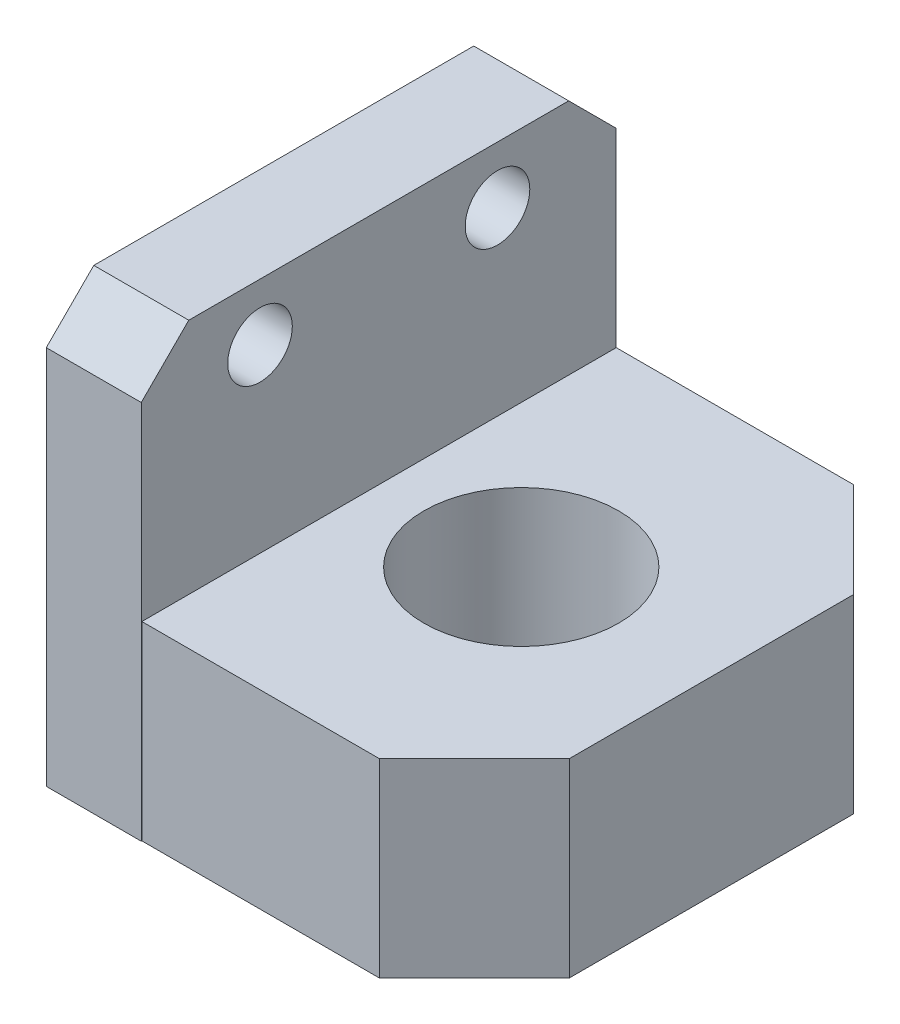
SolidWorks part; units mm, degrees
ref_plane "前视基准面" through (0, 0, 0) normal (0, 0, 1) x (1, 0, 0)
ref_plane "上视基准面" through (0, 0, 0) normal (0, 1, 0) x (1, 0, 0)
ref_plane "右视基准面" through (0, 0, 0) normal (1, 0, 0) x (0, 0, -1)
sketch "草图1" plane through (0, 0, 0) normal (1, 0, 0) x (0, 0, -1)
  line L1 (-25, 22.5) -> (25, 22.5)
  line L2 (-25, 22.5) -> (-25, -22.5)
  line L3 (-25, -22.5) -> (25, -22.5)
  line L4 (25, 22.5) -> (25, -22.5)
  line L5 (-25, 22.5) -> (25, -22.5) construction
  line L6 (-25, -22.5) -> (25, 22.5) construction
  point P0 (0, 0)
  dimension "D1" = 50
  dimension "D2" = 45
extrude "凸台-拉伸1" add sketch "草图1" along normal blind 10
sketch "草图2" plane through (10, 0, 0) normal (1, 0, 0) x (0, 0, -1)
  line L0 (25, -22.5) -> (25, 22.5) construction
  line L1 (-24.9382, -2.5) -> (25, -2.5)
  line L2 (-24.9382, -2.5) -> (-24.9382, -22.5)
  line L3 (-24.9382, -22.5) -> (25, -22.5)
  line L4 (25, -2.5) -> (25, -22.5)
  line L5 (-24.9382, -2.5) -> (25, -22.5) construction
  line L6 (-24.9382, -22.5) -> (25, -2.5) construction
  line L7 (-25, -22.5) -> (25, -22.5) construction
  dimension "D2" = 20
extrude "凸台-拉伸2" add sketch "草图2" along normal blind 35
hole_wizard "Ø20.5 (20.5) 直径孔1" positions "草图3" profile "草图4" hole size "Ø20.5" standard "GB" end condition through all
sketch "草图3" plane through (0, -22.5, 0) normal (0, -1, 0) x (-1, 0, 0)
  point P0 (-25, 0)
  dimension "D1" = 25
sketch "草图4" plane through (25, -22.5, 0) normal (1, 0, 0) x (0, 0, -1)
  line L0 (0, 0) -> (0, 45)
  line L1 (0, 45) -> (10.25, 45)
  line L2 (10.25, 45) -> (10.25, 0)
  line L5 (10.25, 0) -> (0, 0)
  line L11 (0, -6.35) -> (0, 107.95) construction
  dimension "通孔孔直径" = 20.5
  dimension "通孔孔深度" = 45
hole_wizard "M8 螺纹孔1" positions "草图5" profile "草图6" tap size "M8" standard "GB"
sketch "草图5" plane through (10, 0, 0) normal (1, 0, 0) x (0, 0, -1)
  line L0 (0, 27.2455) -> (0, 0) construction
  line L2 (25, 22.5) -> (-25, 22.5) construction
  point P0 (-12.5, 16.5)
  point P2 (12.5, 16.5)
  point P4 (-12.5, -13.5)
  point P6 (12.5, -13.5)
  dimension "D1" = 25
  dimension "D2" = 30
  dimension "D3" = 6
sketch "草图6" plane through (10, 16.5, 12.5) normal (0, 1, 0) x (0, 0, -1)
  line L0 (0, 0) -> (0, 10)
  line L1 (0, 10) -> (3.4, 10)
  line L2 (3.4, 10) -> (3.4, 0)
  line L5 (3.4, 0) -> (0, 0)
  line L11 (0, -6.35) -> (0, 107.95) construction
  dimension "通孔螺纹孔钻头直径" = 6.8
  dimension "通孔螺纹孔钻头深度" = 10
cosmetic thread "孔螺蚊线1" parameters "D2"=8
cosmetic thread "孔螺蚊线2" parameters "D2"=8
cosmetic thread "孔螺蚊线3" parameters "D2"=8
cosmetic thread "孔螺蚊线4" parameters "D2"=8
chamfer "倒角1" distance 10 angle 45 2 edges at (45, -12.5, -25) (45, -12.5, 24.9382)
chamfer "倒角2" distance 5 angle 45 2 edges at (5, 22.5, -25) (5, 22.5, 25)
